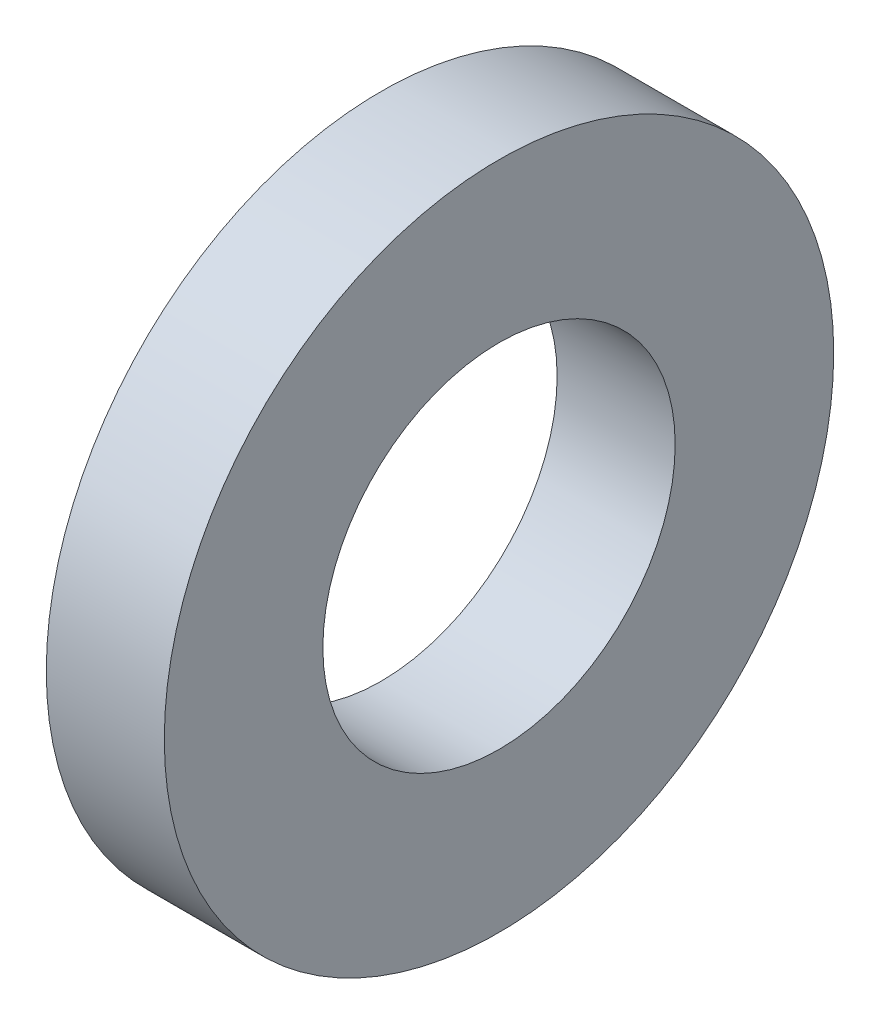
SolidWorks part; units mm, degrees
ref_plane "Front Plane" through (0, 0, 0) normal (0, 0, 1) x (1, 0, 0)
ref_plane "Top Plane" through (0, 0, 0) normal (0, 1, 0) x (1, 0, 0)
ref_plane "Right Plane" through (0, 0, 0) normal (1, 0, 0) x (0, 0, -1)
sketch "Sketch1" plane through (0, 0, 0) normal (1, 0, 0) x (0, 0, -1)
  circle A0 centre (0, 0) radius 10
  circle A1 centre (0, 0) radius 19
  dimension "D1" = 20
  dimension "D2" = 38
extrude "Boss-Extrude1" add sketch "Sketch1" along normal blind 6.7
